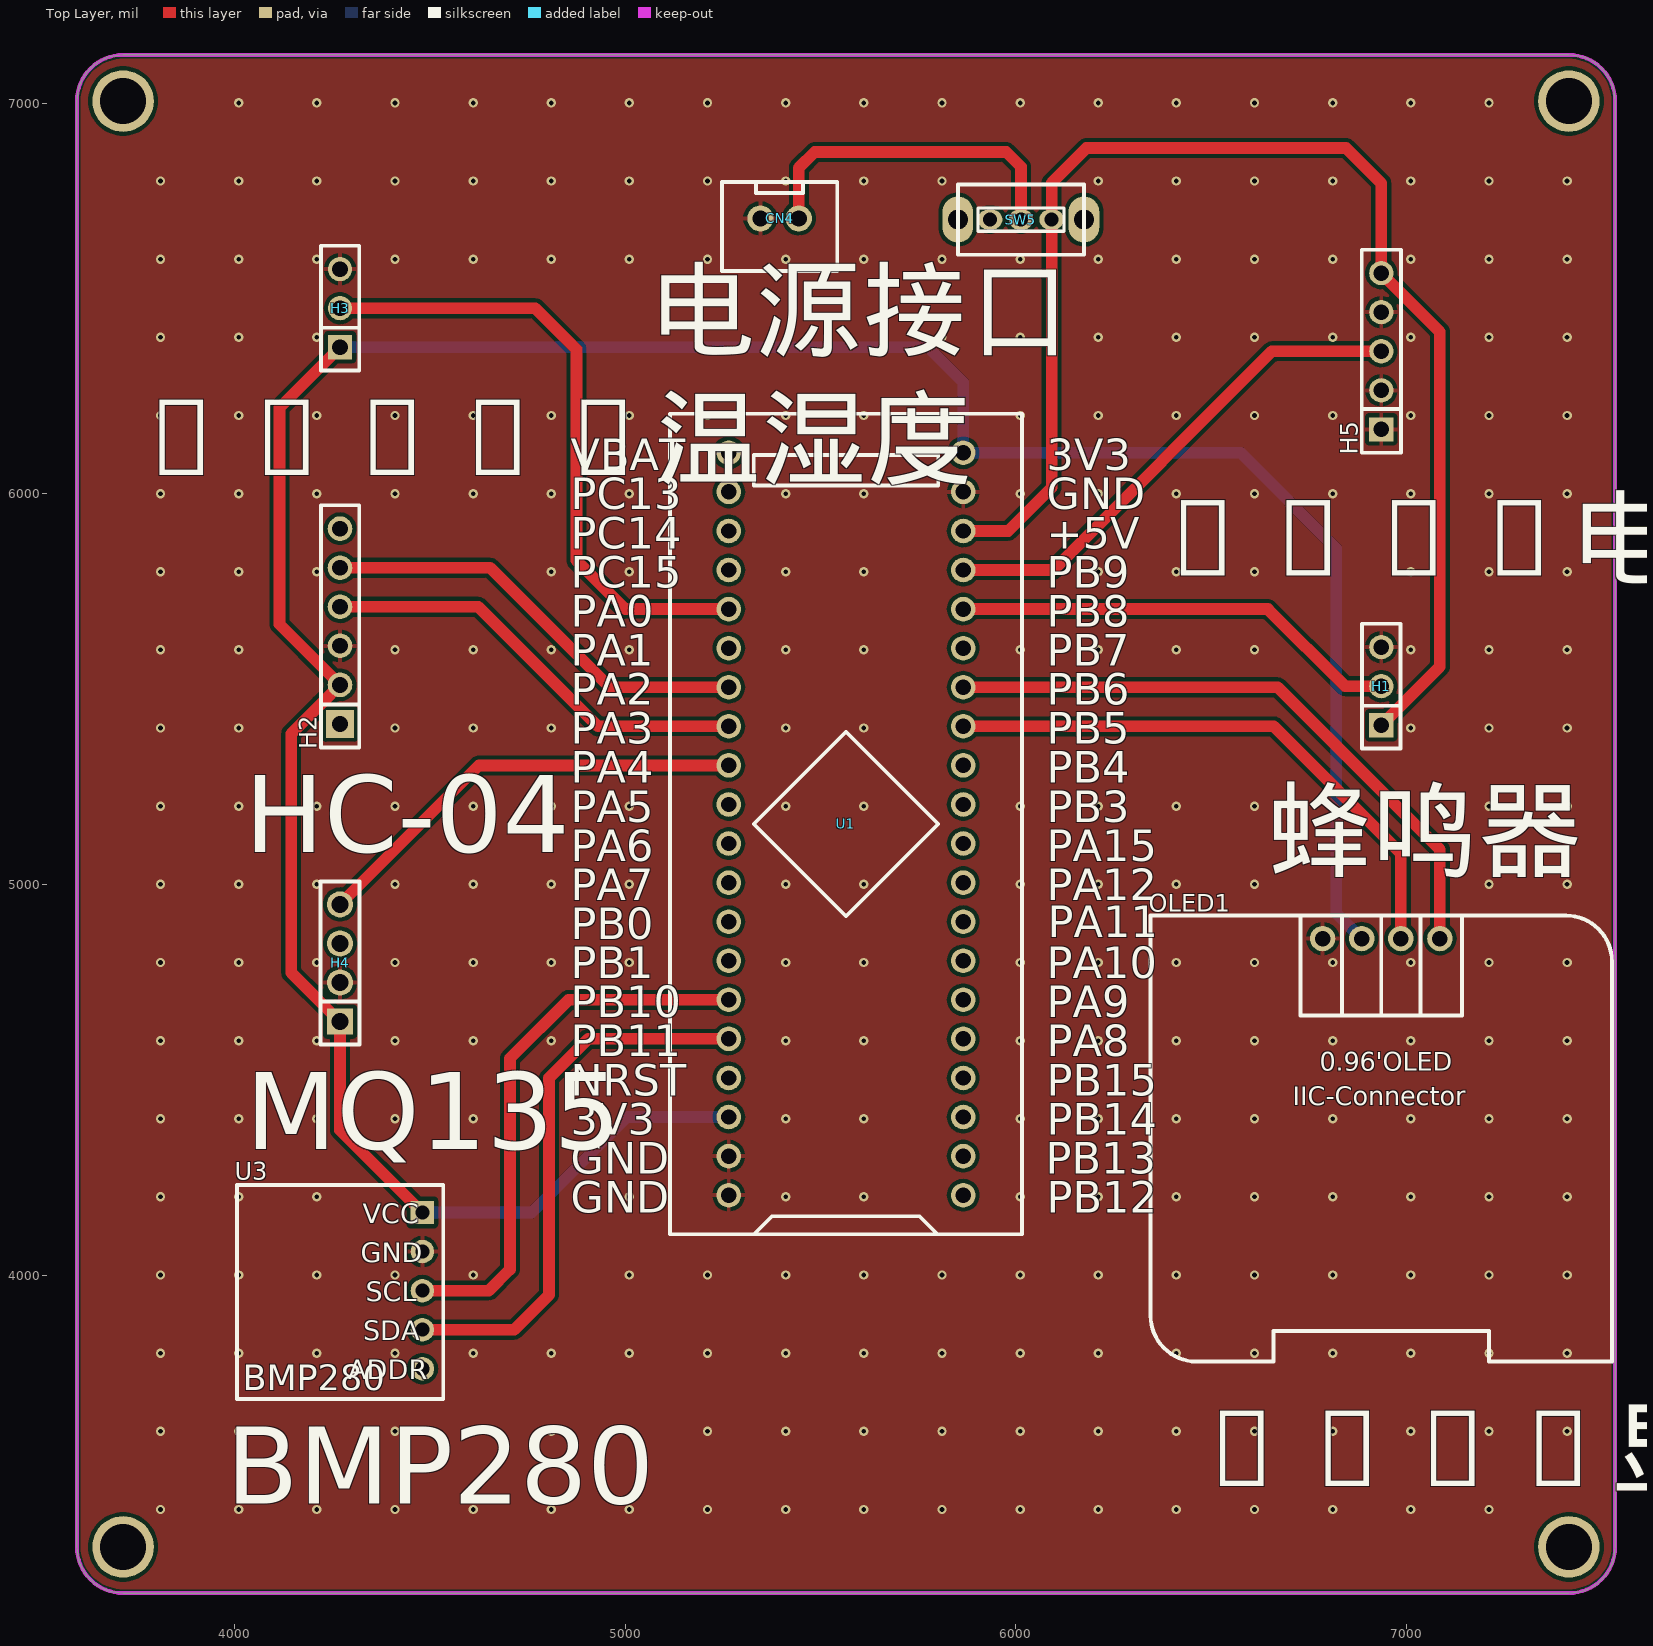
[diagram p0: Top Layer view]
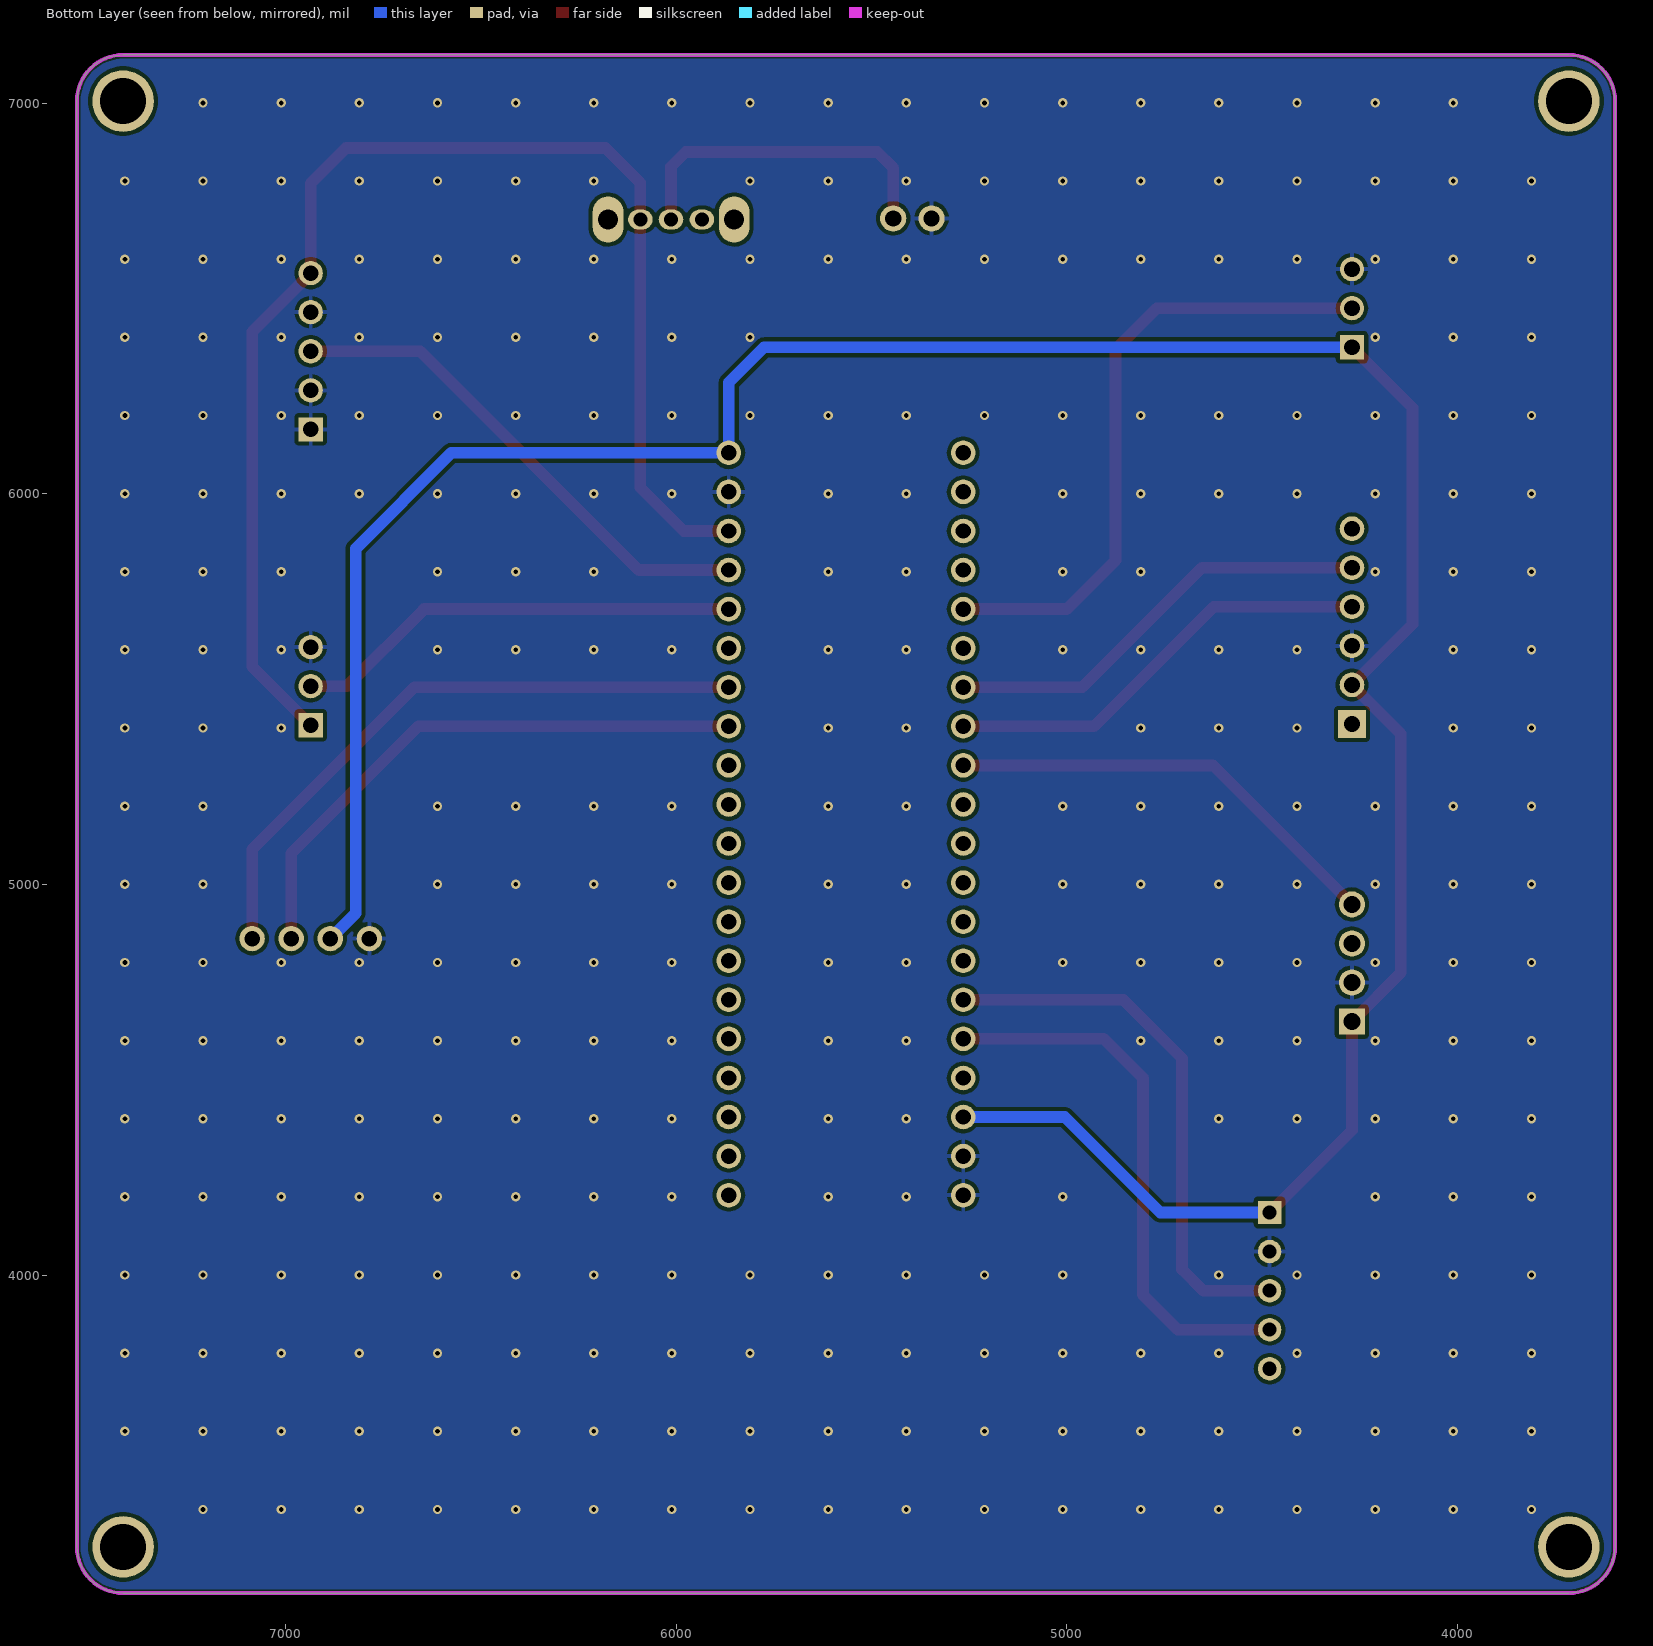
[diagram p1: Bottom Layer view, seen from below]
# Altium PCB MISC51936.pcbdoc
Units mil, origin at the board's own origin, x right, y up, seen from the top; angles counter-clockwise.
Board outline 3937.01 x 3937.01 mil, 2 copper layers (Top Layer, Bottom Layer), stack 62.206 mil thick; 10 components, 38 nets, 81 pads, 306 vias.

## Layer stack, top to bottom
Top Solder Mask Layer: solder mask 0.394, Dk 3.3
Top Layer: signal copper 1.379
Dielectric1: surface 59.449, FR4, Dk 4.5
Bottom Layer: signal copper 1.378
Bottom Solder Mask Layer: solder mask 0.394, Dk 3.3

## Board outline
3714.61,7123.5 ccw(c3714.61,7005.39) 3596.5,7005.39 3596.5,3304.61 ccw(c3714.61,3304.61) 3714.61,3186.5 7415.39,3186.5 ccw(c7415.39,3304.61) 7533.5,3304.61 7533.5,7005.39 ccw(c7415.39,7005.39) 7415.39,7123.5 3714.61,7123.5

## Design rules (kind name [scope] priority, off if disabled: settings)
BoardOutlineClearance copperThickness2oz_1 [All] p2 off: genericclearance=7.99 ignorepadtopadclearanceinfootprint=FALSE except(0: Arc-SplitContinuation Track-SplitContinuation SMDPad-SplitContinuation THPad-SplitContinuation Via-SplitContinuation Fill-SplitContinuation Region-SplitContinuation Poly-SplitContinuation Text-SplitContinuation Hole-SplitContinuation; 5.98: Arc-CutoutEdge Track-CutoutEdge SMDPad-CutoutEdge THPad-CutoutEdge Via-CutoutEdge Text-CutoutEdge; 6.9: Hole-OutlineEdge Hole-CutoutEdge; 10: Poly-OutlineEdge Poly-CutoutEdge; 11.81: Arc-OutlineEdge Track-OutlineEdge SMDPad-OutlineEdge THPad-OutlineEdge Via-OutlineEdge Fill-OutlineEdge Region-OutlineEdge Text-OutlineEdge Fill-CutoutEdge Region-CutoutEdge)
BoardOutlineClearance Plane_innerPlane_1 [All] p4 off: genericclearance=4.02 ignorepadtopadclearanceinfootprint=FALSE except(0: Arc-SplitContinuation Track-SplitContinuation SMDPad-SplitContinuation THPad-SplitContinuation Via-SplitContinuation Fill-SplitContinuation Region-SplitContinuation Poly-SplitContinuation Text-SplitContinuation Hole-SplitContinuation; 5.98: Arc-CutoutEdge Track-CutoutEdge SMDPad-CutoutEdge THPad-CutoutEdge Via-CutoutEdge Text-CutoutEdge; 6.9: Hole-OutlineEdge Hole-CutoutEdge; 10: Poly-OutlineEdge Poly-CutoutEdge; 11.81: Arc-OutlineEdge Track-OutlineEdge SMDPad-OutlineEdge THPad-OutlineEdge Via-OutlineEdge Fill-OutlineEdge Region-OutlineEdge Text-OutlineEdge Fill-CutoutEdge Region-CutoutEdge)
BoardOutlineClearance Copper_copperRegion_1 [All] p6 off: genericclearance=4.02 ignorepadtopadclearanceinfootprint=FALSE except(0: Arc-SplitContinuation Track-SplitContinuation SMDPad-SplitContinuation THPad-SplitContinuation Via-SplitContinuation Fill-SplitContinuation Region-SplitContinuation Poly-SplitContinuation Text-SplitContinuation Hole-SplitContinuation; 5.98: Arc-CutoutEdge Track-CutoutEdge SMDPad-CutoutEdge THPad-CutoutEdge Via-CutoutEdge Text-CutoutEdge; 6.9: Hole-OutlineEdge Hole-CutoutEdge; 10: Poly-OutlineEdge Poly-CutoutEdge; 11.81: Arc-OutlineEdge Track-OutlineEdge SMDPad-OutlineEdge THPad-OutlineEdge Via-OutlineEdge Fill-OutlineEdge Region-OutlineEdge Text-OutlineEdge Fill-CutoutEdge Region-CutoutEdge)
BoardOutlineClearance Copper_copperRegion_copperThickness1oz_1 [All] p8 off: genericclearance=4.02 ignorepadtopadclearanceinfootprint=FALSE except(0: Arc-SplitContinuation Track-SplitContinuation SMDPad-SplitContinuation THPad-SplitContinuation Via-SplitContinuation Fill-SplitContinuation Region-SplitContinuation Poly-SplitContinuation Text-SplitContinuation Hole-SplitContinuation; 5.98: Arc-CutoutEdge Track-CutoutEdge SMDPad-CutoutEdge THPad-CutoutEdge Via-CutoutEdge Text-CutoutEdge; 6.9: Hole-OutlineEdge Hole-CutoutEdge; 10: Poly-OutlineEdge Poly-CutoutEdge; 11.81: Arc-OutlineEdge Track-OutlineEdge SMDPad-OutlineEdge THPad-OutlineEdge Via-OutlineEdge Fill-OutlineEdge Region-OutlineEdge Text-OutlineEdge Fill-CutoutEdge Region-CutoutEdge)
BoardOutlineClearance Copper_copperRegion_Copper_copperRegion_1 [All] p10 off: genericclearance=4.02 ignorepadtopadclearanceinfootprint=FALSE except(0: Arc-SplitContinuation Track-SplitContinuation SMDPad-SplitContinuation THPad-SplitContinuation Via-SplitContinuation Fill-SplitContinuation Region-SplitContinuation Poly-SplitContinuation Text-SplitContinuation Hole-SplitContinuation; 5.98: Arc-CutoutEdge Track-CutoutEdge SMDPad-CutoutEdge THPad-CutoutEdge Via-CutoutEdge Text-CutoutEdge; 6.9: Hole-OutlineEdge Hole-CutoutEdge; 10: Poly-OutlineEdge Poly-CutoutEdge; 11.81: Arc-OutlineEdge Track-OutlineEdge SMDPad-OutlineEdge THPad-OutlineEdge Via-OutlineEdge Fill-OutlineEdge Region-OutlineEdge Text-OutlineEdge Fill-CutoutEdge Region-CutoutEdge)
BoardOutlineClearance copperThickness1oz_1 [All] p12: genericclearance=4.02 ignorepadtopadclearanceinfootprint=FALSE except(0: Arc-SplitContinuation Track-SplitContinuation SMDPad-SplitContinuation THPad-SplitContinuation Via-SplitContinuation Fill-SplitContinuation Region-SplitContinuation Poly-SplitContinuation Text-SplitContinuation Hole-SplitContinuation; 5.98: Arc-CutoutEdge Track-CutoutEdge SMDPad-CutoutEdge THPad-CutoutEdge Via-CutoutEdge Text-CutoutEdge; 6.9: Hole-OutlineEdge Hole-CutoutEdge; 10: Poly-OutlineEdge Poly-CutoutEdge; 11.81: Arc-OutlineEdge Track-OutlineEdge SMDPad-OutlineEdge THPad-OutlineEdge Via-OutlineEdge Fill-OutlineEdge Region-OutlineEdge Text-OutlineEdge Fill-CutoutEdge Region-CutoutEdge)
Clearance copperThickness2oz [All] p1 off: gap=7.99 ignorepadtopadclearanceinfootprint=FALSE except(5.98: SMDPad-Track SMDPad-SMDPad THPad-Track SMDPad-THPad THPad-THPad Track-Via SMDPad-Via THPad-Via Via-Via Fill-SMDPad Region-SMDPad Fill-THPad Region-THPad Fill-Via Region-Via Fill-Fill Fill-Region Region-Region Arc-Track Arc-SMDPad Arc-THPad Arc-Via Fill-Arc Region-Arc Arc-Arc Text-Track SMDPad-Text Text-THPad Text-Via Fill-Text Region-Text Arc-Text Text-Text; 6.9: Hole-Track Hole-SMDPad Hole-THPad Hole-Via Fill-Hole Region-Hole Hole-Arc Hole-Text; 10: Poly-Track Poly-SMDPad Poly-THPad Poly-Via Poly-Fill Poly-Region Poly-Poly Poly-Arc Poly-Text Poly-Hole; 11.81: Fill-Track Region-Track)
Clearance Plane_innerPlane [All] p3 off: gap=4.02 ignorepadtopadclearanceinfootprint=FALSE except(5.98: SMDPad-Track SMDPad-SMDPad THPad-Track SMDPad-THPad THPad-THPad Track-Via SMDPad-Via THPad-Via Via-Via Fill-SMDPad Region-SMDPad Fill-THPad Region-THPad Fill-Via Region-Via Fill-Fill Fill-Region Region-Region Arc-Track Arc-SMDPad Arc-THPad Arc-Via Fill-Arc Region-Arc Arc-Arc Text-Track SMDPad-Text Text-THPad Text-Via Fill-Text Region-Text Arc-Text Text-Text; 6.9: Hole-Track Hole-SMDPad Hole-THPad Hole-Via Fill-Hole Region-Hole Hole-Arc Hole-Text; 10: Poly-Track Poly-SMDPad Poly-THPad Poly-Via Poly-Fill Poly-Region Poly-Poly Poly-Arc Poly-Text Poly-Hole; 11.81: Fill-Track Region-Track)
Clearance Copper_copperRegion [All] p5 off: gap=4.02 ignorepadtopadclearanceinfootprint=FALSE except(5.98: SMDPad-Track SMDPad-SMDPad THPad-Track SMDPad-THPad THPad-THPad Track-Via SMDPad-Via THPad-Via Via-Via Fill-SMDPad Region-SMDPad Fill-THPad Region-THPad Fill-Via Region-Via Fill-Fill Fill-Region Region-Region Arc-Track Arc-SMDPad Arc-THPad Arc-Via Fill-Arc Region-Arc Arc-Arc Text-Track SMDPad-Text Text-THPad Text-Via Fill-Text Region-Text Arc-Text Text-Text; 6.9: Hole-Track Hole-SMDPad Hole-THPad Hole-Via Fill-Hole Region-Hole Hole-Arc Hole-Text; 10: Poly-Track Poly-SMDPad Poly-THPad Poly-Via Poly-Fill Poly-Region Poly-Poly Poly-Arc Poly-Text Poly-Hole; 11.81: Fill-Track Region-Track)
Clearance Copper_copperRegion_copperThickness1oz [All] p7 off: gap=4.02 ignorepadtopadclearanceinfootprint=FALSE except(5.98: SMDPad-Track SMDPad-SMDPad THPad-Track SMDPad-THPad THPad-THPad Track-Via SMDPad-Via THPad-Via Via-Via Fill-SMDPad Region-SMDPad Fill-THPad Region-THPad Fill-Via Region-Via Fill-Fill Fill-Region Region-Region Arc-Track Arc-SMDPad Arc-THPad Arc-Via Fill-Arc Region-Arc Arc-Arc Text-Track SMDPad-Text Text-THPad Text-Via Fill-Text Region-Text Arc-Text Text-Text; 6.9: Hole-Track Hole-SMDPad Hole-THPad Hole-Via Fill-Hole Region-Hole Hole-Arc Hole-Text; 10: Poly-Track Poly-SMDPad Poly-THPad Poly-Via Poly-Fill Poly-Region Poly-Poly Poly-Arc Poly-Text Poly-Hole; 11.81: Fill-Track Region-Track)
Clearance Copper_copperRegion_Copper_copperRegion [All] p9 off: gap=4.02 ignorepadtopadclearanceinfootprint=FALSE except(5.98: SMDPad-Track SMDPad-SMDPad THPad-Track SMDPad-THPad THPad-THPad Track-Via SMDPad-Via THPad-Via Via-Via Fill-SMDPad Region-SMDPad Fill-THPad Region-THPad Fill-Via Region-Via Fill-Fill Fill-Region Region-Region Arc-Track Arc-SMDPad Arc-THPad Arc-Via Fill-Arc Region-Arc Arc-Arc Text-Track SMDPad-Text Text-THPad Text-Via Fill-Text Region-Text Arc-Text Text-Text; 6.9: Hole-Track Hole-SMDPad Hole-THPad Hole-Via Fill-Hole Region-Hole Hole-Arc Hole-Text; 10: Poly-Track Poly-SMDPad Poly-THPad Poly-Via Poly-Fill Poly-Region Poly-Poly Poly-Arc Poly-Text Poly-Hole; 11.81: Fill-Track Region-Track)
Clearance copperThickness1oz [All] p11: gap=4.02 ignorepadtopadclearanceinfootprint=FALSE except(5.98: SMDPad-Track SMDPad-SMDPad THPad-Track SMDPad-THPad THPad-THPad Track-Via SMDPad-Via THPad-Via Via-Via Fill-SMDPad Region-SMDPad Fill-THPad Region-THPad Fill-Via Region-Via Fill-Fill Fill-Region Region-Region Arc-Track Arc-SMDPad Arc-THPad Arc-Via Fill-Arc Region-Arc Arc-Arc Text-Track SMDPad-Text Text-THPad Text-Via Fill-Text Region-Text Arc-Text Text-Text; 6.9: Hole-Track Hole-SMDPad Hole-THPad Hole-Via Fill-Hole Region-Hole Hole-Arc Hole-Text; 10: Poly-Track Poly-SMDPad Poly-THPad Poly-Via Poly-Fill Poly-Region Poly-Poly Poly-Arc Poly-Text Poly-Hole; 11.81: Fill-Track Region-Track)
DiffPairsRouting differentialPair [All] p1: maxlimit=6 minlimit=6 mostfreqgap=6 toplayer_minwidth=5 toplayer_prefwidth=10 toplayer_maxwidth=100 toplayer_mingap=6 toplayer_prefgap=6 toplayer_maxgap=6 bottomlayer_minwidth=5 bottomlayer_prefwidth=10 bottomlayer_maxwidth=100 bottomlayer_mingap=6 bottomlayer_prefgap=6 bottomlayer_maxgap=6 maxuncoupledlength=10
HoleToHoleClearance otherClearance [All] p1: gap=11.81 allowstackedmicrovias=TRUE
Length netLength [All] p1: minlimit=0 maxlimit=0
PasteMaskExpansion pasteMaskExpansion [All] p1: expansion=0
PlaneConnect innerPlane [All] p1: planeconnectstyle=Relief reliefexpansion=20 reliefentries=4 reliefconductorwidth=10 reliefairgap=10
PolygonConnect copperRegion_copperThickness1oz [All] p1 off: connectstyle=Relief reliefconductorwidth=10 reliefentries=4 polygonreliefangle="90 Angle" airgapwidth=10 via.connectstyle=Relief via.reliefconductorwidth=10 via.reliefentries=4 via.polygonreliefangle="90 Angle" via.airgapwidth=10
PolygonConnect copperRegion_Copper_copperRegion [All] p2 off: connectstyle=Relief reliefconductorwidth=10 reliefentries=4 polygonreliefangle="90 Angle" airgapwidth=10 via.connectstyle=Relief via.reliefconductorwidth=10 via.reliefentries=4 via.polygonreliefangle="90 Angle" via.airgapwidth=10
PolygonConnect copperRegion [All] p3: connectstyle=Relief reliefconductorwidth=10 reliefentries=4 polygonreliefangle="90 Angle" airgapwidth=10 via.connectstyle=Relief via.reliefconductorwidth=10 via.reliefentries=4 via.polygonreliefangle="90 Angle" via.airgapwidth=10
RoutingVias viaSize [All] p1: holewidth=12.01 width=24.02 viastyle="Through Hole" minholewidth=11.81 minwidth=19.68 maxholewidth=248.03 maxwidth=393.7
SolderMaskExpansion solderMaskExpansion [IsVia] p1: expansion=-1000 istentingtop=TRUE
SolderMaskExpansion solderMaskExpansion [All] p2: expansion=2 istentingtop=FALSE
Width copperThickness2oz_2 [All] p1 off: maxlimit=100 minlimit=8 preferedwidth=10
Width copperThickness1oz_2 [All] p2: maxlimit=100 minlimit=5 preferedwidth=10

## Components (designator, comment, footprint, x,y, rotation, side; value= is the part's Value field where it differs from the comment)
CN4 "XH2.54*2P_直插" CONN-TH_2P-P2.50-XH2.54-2P 5395,6705 r0 top
H1 "" HDR-TH_3P-P2.54-V-F 6935,5507.64 r90 top
H2 "" HDR-TH_6P-P2.54-V-F 4270,5660.97 r90 top
H3 "" HDR-TH_3P-P2.54-V-F 4270,6475.16 r90 top
H4 "" HDR-TH_4P-P2.54-V-F 4270,4799.26 r90 top
H5 "" HDR-TH_5P-P2.54-V-F 6935,6365 r90 top
OLED1 "" 0.96OLED_4P 6935,4861.7 r0 top
SW5 "" 拨动开关 6017.9,6702.05 r180 top
U1 "STM32F103C8T6-Card" CONN-TH_L53.3-W22.9_STM32F103C8T6-CARD 5565,5155 r90 top
U3 "" BH1750光照传感器 4220.83,3950.68 r0 top

## Footprints (in the part's own frame and the unit in brackets; to place one, negate y for a bottom-side part, rotate by r counter-clockwise, add the part's x,y. Pads: shape width x height; smd on the part's side, far side on the other; paste and mask are expansions set on the pad)
0.96OLED_4P [mm]
  round 1.65 hole 1 copper offset 0,0: 1(-3.81,-0.001) 2(-1.27,0.002) 3(1.27,0.002) 4(3.81,0.002)
  silkscreen extent -15,-27.5 15,1.5
BH1750光照传感器 [mil]
  rect 60x60 hole 36: 1(260,210)
  round 60 hole 36: 2(260,110) 3(260,10) 4(260,-90) 5(260,-190)
  silkscreen extent -215,-267 313,280
CONN-TH_2P-P2.50-XH2.54-2P [mm]
  round 1.7 hole 1.05 paste+0 mask+0.05: 1(1.25,0) 2(-1.25,0)
  silkscreen extent -3.75,-3.42 3.75,2.37
CONN-TH_L53.3-W22.9_STM32F103C8T6-CARD [mm]
  round 1.6 hole 1: 1(-24.13,-7.62) 2(-21.59,-7.62) 3(-19.05,-7.62) 4(-16.51,-7.62) 5(-13.97,-7.62) 6(-11.43,-7.62) 7(-8.89,-7.62) 8(-6.35,-7.62) 9(-3.81,-7.62) 10(-1.27,-7.62) 11(1.27,-7.62) 12(3.81,-7.62) 13(6.35,-7.62) 14(8.89,-7.62) 15(11.43,-7.62) 16(13.97,-7.62) 17(16.51,-7.62) 18(19.05,-7.62) 19(21.59,-7.62) 20(24.13,-7.62) 21(24.13,7.62) 22(21.59,7.62) 23(19.05,7.62) 24(16.51,7.62) 25(13.97,7.62) 26(11.43,7.62) 27(8.89,7.62) 28(6.35,7.62) 29(3.81,7.62) 30(1.27,7.62) 31(-1.27,7.62) 32(-3.81,7.62) 33(-6.35,7.62) 34(-8.89,7.62) 35(-11.43,7.62) 36(-13.97,7.62) 37(-16.51,7.62) 38(-19.05,7.62) 39(-21.59,7.62) 40(-24.13,7.62)
  silkscreen extent -26.67,-11.43 26.67,11.43
HDR-TH_3P-P2.54-V-F [mil]
  rect 62x62 hole 40.16: 1(-100,0)
  round 62 hole 40.16: 2(0,0) 3(100,0)
  silkscreen extent -160,-49 160,49
HDR-TH_4P-P2.54-V-F [mm]
  rect 1.7x1.7 hole 1.1: 1(-3.81,0)
  round 1.7 hole 1.1: 2(-1.27,0) 3(1.27,0) 4(3.81,0)
  silkscreen extent -5.29,-1.27 5.29,1.27
HDR-TH_5P-P2.54-V-F [mil]
  rect 62x62 hole 40.16: 1(-200,0)
  round 62 hole 40.16: 2(-100,0) 3(0,0) 4(100,0) 5(200,0)
  silkscreen extent -260,-50 260,50
HDR-TH_6P-P2.54-V-F [mm]
  rect 1.8x1.8 hole 1.02: 1(-6.35,0)
  round 1.6 hole 1.02: 2(-3.81,0) 3(-1.27,0) 4(1.27,0) 5(3.81,0) 6(6.35,0)
  silkscreen extent -7.87,-1.25 7.87,1.25
拨动开关 [mil]
  oval 63x51.2 hole 35.4 paste+0 mask+2: 1(-73.4,0) 2(5,0) 3(84,0)
  oval 78.7x118.1 hole 51.2 paste+0 mask+2: 4(166.7,0) 5(-156.1,0)
  silkscreen extent -156,-90 167,90

## Free pads (board coordinates)
  round 157.48 hole 118.11: 1(3714.61,7005.39) 1(3714.61,3304.61) 1(7415.39,7005.39) 1(7415.39,3304.61)

## Via types
v1: diameter 24.02, hole 12, Top Layer to Bottom Layer, 306 vias

## Nets (pads, with @x,y where several pads share a name; then routed paths per layer and width w, separated by ;. In a path a pad name is that pad's centre, name@x,y a point inside that pad or via, vN(x,y) a via of type N, cw(c..) or ccw(c..) an arc to the next point about the centre after c; other vN are vias at no path point)
$1N17118: CN4.1 SW5.2 | length 865.5
  Top Layer w30: CN4.1 5444.22,6834.22 5485,6875 5975,6875 6012.9,6837.1 SW5.2
+5V: H1.1 H5.5 SW5.1 U1.18 | length 3481.8
  Top Layer w30: U1.18 5980,5905 6091.3,6016.3 SW5.1 6091.3,6796.3 6180,6885 6845,6885 6935,6795 H5.5 7085,6415 7085,5557.64 H1.1
GND: CN4.2 H1.3 H2.3 H3.3 H4.2 H5.1 H5.2 H5.4 OLED1.1 U1.19 U1.39 U1.40 U3.2
  other v1: 3810.6,3400.6 4010.6,3400.6 4210.6,3400.6 4410.6,3400.6 4610.6,3400.6 4810.6,3400.6 5010.6,3400.6 5210.6,3400.6 5410.6,3400.6 5610.6,3400.6 5810.6,3400.6 6010.6,3400.6 6210.6,3400.6 6410.6,3400.6 6610.6,3400.6 6810.6,3400.6 7010.6,3400.6 7210.6,3400.6 3810.6,3600.6 4010.6,3600.6 4210.6,3600.6 4410.6,3600.6 4610.6,3600.6 4810.6,3600.6 5010.6,3600.6 5210.6,3600.6 5410.6,3600.6 5610.6,3600.6 5810.6,3600.6 6010.6,3600.6 6210.6,3600.6 6410.6,3600.6 6610.6,3600.6 6810.6,3600.6 7010.6,3600.6 7210.6,3600.6 7410.6,3600.6 3810.6,3800.6 4010.6,3800.6 4210.6,3800.6 4410.6,3800.6 4610.6,3800.6 4810.6,3800.6 5010.6,3800.6 5210.6,3800.6 5410.6,3800.6 5610.6,3800.6 5810.6,3800.6 6010.6,3800.6 6210.6,3800.6 6410.6,3800.6 6610.6,3800.6 6810.6,3800.6 7010.6,3800.6 7210.6,3800.6 7410.6,3800.6 3810.6,4000.6 4010.6,4000.6 4210.6,4000.6 4410.6,4000.6 4610.6,4000.6 5010.6,4000.6 5210.6,4000.6 5410.6,4000.6 5610.6,4000.6 5810.6,4000.6 6010.6,4000.6 6210.6,4000.6 6410.6,4000.6 6610.6,4000.6 6810.6,4000.6 7010.6,4000.6 7210.6,4000.6 7410.6,4000.6 3810.6,4200.6 4010.6,4200.6 4210.6,4200.6 5010.6,4200.6 5410.6,4200.6 5610.6,4200.6 6010.6,4200.6 6210.6,4200.6 6410.6,4200.6 6610.6,4200.6 6810.6,4200.6 7010.6,4200.6 7210.6,4200.6 7410.6,4200.6 3810.6,4400.6 4010.6,4400.6 4210.6,4400.6 4410.6,4400.6 4610.6,4400.6 5410.6,4400.6 5610.6,4400.6 6010.6,4400.6 6210.6,4400.6 6410.6,4400.6 6610.6,4400.6 6810.6,4400.6 7010.6,4400.6 7210.6,4400.6 7410.6,4400.6 3810.6,4600.6 4010.6,4600.6 4210.6,4600.6 4410.6,4600.6 4610.6,4600.6 4810.6,4600.6 5410.6,4600.6 5610.6,4600.6 6010.6,4600.6 6210.6,4600.6 6410.6,4600.6 6610.6,4600.6 6810.6,4600.6 7010.6,4600.6 7210.6,4600.6 7410.6,4600.6 3810.6,4800.6 4010.6,4800.6 4210.6,4800.6 4410.6,4800.6 4610.6,4800.6 4810.6,4800.6 5010.6,4800.6 5410.6,4800.6 5610.6,4800.6 6010.6,4800.6 6210.6,4800.6 6410.6,4800.6 6610.6,4800.6 6810.6,4800.6 7010.6,4800.6 7210.6,4800.6 7410.6,4800.6 3810.6,5000.6 4010.6,5000.6 4210.6,5000.6 4410.6,5000.6 4610.6,5000.6 4810.6,5000.6 5010.6,5000.6 5410.6,5000.6 5610.6,5000.6 6010.6,5000.6 6210.6,5000.6 6410.6,5000.6 6610.6,5000.6 7210.6,5000.6 7410.6,5000.6 3810.6,5200.6 4010.6,5200.6 4210.6,5200.6 4410.6,5200.6 4610.6,5200.6 4810.6,5200.6 5010.6,5200.6 5410.6,5200.6 5610.6,5200.6 6010.6,5200.6 6210.6,5200.6 6410.6,5200.6 6610.6,5200.6 7210.6,5200.6 7410.6,5200.6 3810.6,5400.6 4010.6,5400.6 4410.6,5400.6 4610.6,5400.6 4810.6,5400.6 5410.6,5400.6 5610.6,5400.6 7010.6,5400.6 7210.6,5400.6 7410.6,5400.6 3810.6,5600.6 4010.6,5600.6 4410.6,5600.6 4610.6,5600.6 4810.6,5600.6 5010.6,5600.6 5410.6,5600.6 5610.6,5600.6 6010.6,5600.6 6210.6,5600.6 6410.6,5600.6 6610.6,5600.6 7010.6,5600.6 7210.6,5600.6 7410.6,5600.6 3810.6,5800.6 4010.6,5800.6 4210.6,5800.6 4810.6,5800.6 5010.6,5800.6 5410.6,5800.6 5610.6,5800.6 6210.6,5800.6 6410.6,5800.6 6610.6,5800.6 7010.6,5800.6 7210.6,5800.6 7410.6,5800.6 3810.6,6000.6 4010.6,6000.6 4210.6,6000.6 4410.6,6000.6 4610.6,6000.6 4810.6,6000.6 5010.6,6000.6 5410.6,6000.6 5610.6,6000.6 6010.6,6000.6 6210.6,6000.6 6410.6,6000.6 6610.6,6000.6 6810.6,6000.6 7010.6,6000.6 7210.6,6000.6 7410.6,6000.6 3810.6,6200.6 4010.6,6200.6 4210.6,6200.6 4410.6,6200.6 4610.6,6200.6 4810.6,6200.6 5010.6,6200.6 5210.6,6200.6 5410.6,6200.6 5610.6,6200.6 5810.6,6200.6 6010.6,6200.6 6210.6,6200.6 6410.6,6200.6 6610.6,6200.6 6810.6,6200.6 7010.6,6200.6 7210.6,6200.6 7410.6,6200.6 3810.6,6400.6 4010.6,6400.6 4210.6,6400.6 5810.6,6400.6 6010.6,6400.6 6210.6,6400.6 6410.6,6400.6 6610.6,6400.6 6810.6,6400.6 7010.6,6400.6 7210.6,6400.6 7410.6,6400.6 3810.6,6600.6 4010.6,6600.6 4210.6,6600.6 4410.6,6600.6 4610.6,6600.6 4810.6,6600.6 5010.6,6600.6 5210.6,6600.6 5410.6,6600.6 5610.6,6600.6 5810.6,6600.6 6010.6,6600.6 6210.6,6600.6 6410.6,6600.6 6610.6,6600.6 6810.6,6600.6 7010.6,6600.6 7210.6,6600.6 7410.6,6600.6 3810.6,6800.6 4010.6,6800.6 4210.6,6800.6 4410.6,6800.6 4610.6,6800.6 4810.6,6800.6 5010.6,6800.6 5210.6,6800.6 5410.6,6800.6 5610.6,6800.6 5810.6,6800.6 6210.6,6800.6 6410.6,6800.6 6610.6,6800.6 6810.6,6800.6 7010.6,6800.6 7210.6,6800.6 7410.6,6800.6 4010.6,7000.6 4210.6,7000.6 4410.6,7000.6 4610.6,7000.6 4810.6,7000.6 5010.6,7000.6 5210.6,7000.6 5410.6,7000.6 5610.6,7000.6 5810.6,7000.6 6010.6,7000.6 6210.6,7000.6 6410.6,7000.6 6610.6,7000.6 6810.6,7000.6 7010.6,7000.6 7210.6,7000.6
NRST: U1.37
PA0: H3.2 U1.25 | length 1630.3
  Top Layer w30: H3.2 4769.84,6475.16 4875,6370 4875,5830 5000,5705 U1.25
PA1: U1.26
PA2: H2.5 U1.27 | length 1121.7
  Top Layer w30: H2.5 4654.03,5810.97 4960,5505 U1.27
PA3: H2.4 U1.28 | length 1121.7
  Top Layer w30: H2.4 4624.03,5710.97 4930,5405 U1.28
PA4: H4.4 U1.29 | length 1142.4
  Top Layer w30: H4.4 4625.74,5305 U1.29
PA5: U1.30
PA6: U1.31
PA7: U1.32
PA8: U1.5
PA9: U1.6
PA10: U1.7
PA11: U1.8
PA12: U1.9
PA15: U1.10
PB0: U1.33
PB1: U1.34
PB3: U1.11
PB4: U1.12
PB5: OLED1.3 U1.13 | length 1472.9
  Top Layer w30: U1.13 6660,5405 6985,5080 OLED1.3@6985,4861.75
PB6: OLED1.4 U1.14 | length 1620.2
  Top Layer w30: U1.14 6670,5505 7085,5090 OLED1.4@7085,4861.75
PB7: U1.15
PB8: H1.2 U1.16 | length 1151.7
  Top Layer w30: U1.16 6645,5705 6842.36,5507.64 H1.2
PB9: H5.3 U1.17 | length 1302
  Top Layer w30: U1.17 6095,5805 6655,6365 H5.3
PB10: U1.35 U3.3 | length 1408.8
  Top Layer w30: U3.3 4650.68,3960.68 4705,4015 4705,4555 4855,4705 U1.35
PB11: U1.36 U3.4 | length 1417.6
  Top Layer w30: U3.4 4715.68,3860.68 4805,3950 4805,4505 4905,4605 U1.36
PB12: U1.1
PB13: U1.2
PB14: U1.3
PB15: U1.4
PC13: U1.22
PC14: U1.23
PC15: U1.24
VBAT: U1.21
VCC: H2.2 H3.1 H4.1 OLED1.2 U1.20 U1.38 U3.1 | length 7313.2
  Top Layer w30: H3.1 4115,6220.16 4115,5665.97 H2.2 4222.82,5463.8 ccw(c4234.57,5446.41) 4217.18,5458.15 4145,5385.97 4145,4774.26 H4.1 4270,4371.51 U3.1
  Bottom Layer w30: H3.1 5774.84,6375.16 5865,6285 U1.20 6575,6105 6820,5860 6820,4926.75 OLED1.2@6885,4861.75 ; U3.1 4760.69,4160.69 5005,4405 U1.38
pads on no net: H2.1 H2.6 H4.3 SW5.3 SW5.4 SW5.5 U3.5

## Polygon pours and split planes (outlines as drawn)
GND on Bottom Layer (solid, remove dead copper, pour order 2): 3525,7245 3525,3080 7700,3080 7700,7245
GND on Top Layer (solid, remove dead copper, pour order 2): 3000,7415 3000,3000 7930,3000 7930,7415

## Keep-outs
Board Outline Layer:
  the board outline again, w10

## Silkscreen, mask and mechanical layers (free items; w line width, h text height)
Top Silkscreen Layer:
  text "电源接口" at 5065,6375 h196.85
  text "VBAT" at 4860.95,6060 h80
  text "3V3" at 6079.16,6060 h80
  text "DHT11温湿度" at 3728.66,6047.18 h196.85
  text "PC13" at 4860.95,5960 h80
  text "GND" at 6079.16,5960 h80
  text "PC14" at 4860.95,5860 h80
  text "+5V" at 6079.16,5860 h80
  text "9110电机驱动" at 6344.15,5790.28 h196.85
  text "PC15" at 4860.95,5760 h80
  text "PB9" at 6079.16,5760 h80
  text "PA0" at 4860.95,5660 h80
  text "PB8" at 6079.16,5660 h80
  text "PA1" at 4860.95,5560 h80
  text "PB7" at 6079.16,5560 h80
  text "PA2" at 4860.95,5460 h80
  text "PB6" at 6079.16,5460 h80
  text "PA3" at 4860.95,5360 h80
  text "PB5" at 6079.16,5360 h80
  text "PA4" at 4860.95,5260 h80
  text "PB4" at 6079.16,5260 h80
  text "PA5" at 4860.95,5160 h80
  text "PB3" at 6079.16,5160 h80
  text "HC-04" at 4026.02,5082.69 h196.85
  text "PA6" at 4860.95,5060 h80
  text "PA15" at 6079.16,5060 h80
  text "蜂鸣器" at 6641.81,5042.46 h196.85
  text "PA7" at 4860.95,4960 h80
  text "PA12" at 6079.16,4960 h80
  text "PA11" at 6080.95,4865 h80
  text "PB0" at 4860.95,4860 h80
  text "PB1" at 4860.95,4760 h80
  text "PA10" at 6079.16,4760 h80
  text "PB10" at 4860.95,4660 h80
  text "PA9" at 6079.16,4660 h80
  text "PB11" at 4860.95,4560 h80
  text "PA8" at 6079.16,4560 h80
  text "NRST" at 4860.95,4460 h80
  text "PB15" at 6079.16,4460 h80
  text "3V3" at 4860.95,4360 h80
  text "PB14" at 6079.16,4360 h80
  text "MQ135" at 4029.31,4322.55 h196.85
  text "GND" at 4860.95,4260 h80
  text "PB13" at 6075.95,4260 h80
  text "GND" at 4860.95,4160 h80
  text "PB12" at 6079.16,4160 h80
  text "Oled显示器" at 6443.02,3460 h196.85
  text "BMP280" at 3978.3,3415 h196.85